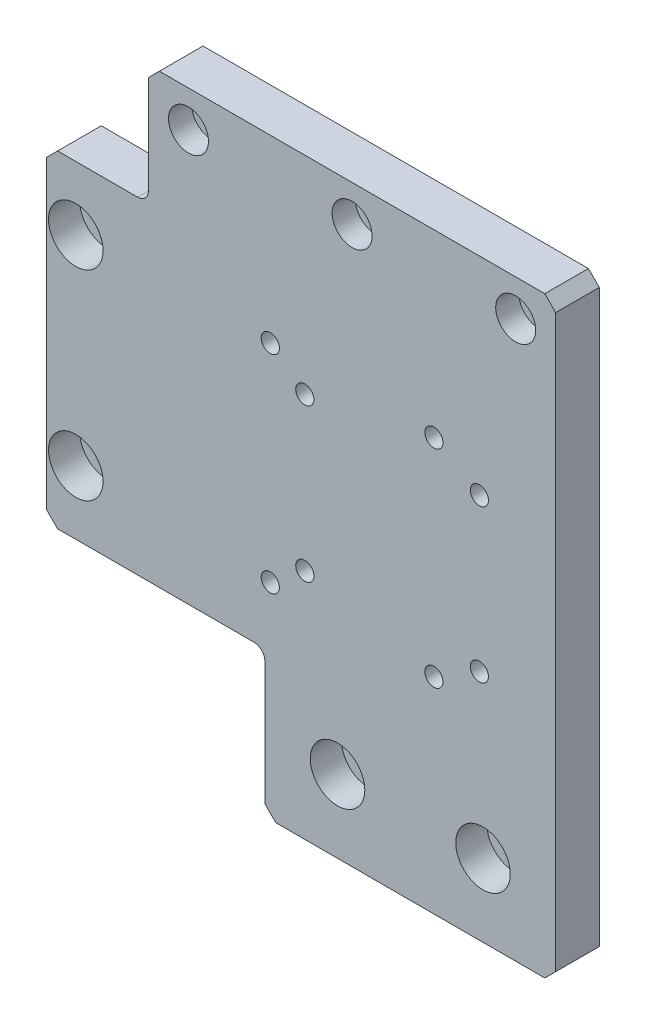
SolidWorks part; units mm, degrees
ref_plane "前视基准面" through (0, 0, 0) normal (0, 0, 1) x (1, 0, 0)
ref_plane "上视基准面" through (0, 0, 0) normal (0, 1, 0) x (1, 0, 0)
ref_plane "右视基准面" through (0, 0, 0) normal (1, 0, 0) x (0, 0, -1)
sketch "草图1" plane through (0, 0, 0) normal (0, 0, 1) x (1, 0, 0)
  line L1 (0, 0) -> (140, 0)
  line L2 (0, 0) -> (0, 112)
  line L3 (0, 112) -> (140, 112)
  line L4 (140, 0) -> (140, 112)
  dimension "D1" = 140
  dimension "D2" = 112
extrude "凸台-拉伸1" add sketch "草图1" along normal blind 12
hole_wizard "M6 螺纹孔1" positions "草图3" profile "草图2" tap size "M6" standard "ISO" end condition through all
sketch "草图3" plane through (0, 0, 0) normal (0, 0, -1) x (-1, 0, 0)
  point P0 (-106.5, 84.5)
  point P8 (-61.5, 84.5)
  point P11 (-61.5, 27.5)
  point P14 (-106.5, 27.5)
sketch "草图2" plane through (106.5, 84.5, 0) normal (1, 0, 0) x (0, 1, 0)
  line L0 (0, 0) -> (0, 12)
  line L1 (0, 12) -> (2.5, 12)
  line L2 (2.5, 12) -> (2.5, 0)
  line L5 (2.5, 0) -> (0, 0)
  line L11 (0, -6.35) -> (0, 107.95) construction
  dimension "通孔螺纹孔钻头直径" = 5
  dimension "通孔螺纹孔钻头深度" = 12
cosmetic thread "孔螺蚊线1" parameters "D2"=6
cosmetic thread "孔螺蚊线2" parameters "D2"=6
cosmetic thread "孔螺蚊线3" parameters "D2"=6
cosmetic thread "孔螺蚊线4" parameters "D2"=6
hole_wizard "M6 螺纹孔2" positions "草图5" profile "草图4" tap size "M6" standard "ISO" end condition through all
sketch "草图5" plane through (0, 0, 12) normal (0, 0, 1) x (1, 0, 0)
  circle A0 centre (119, 77) radius 3.3235 construction
  circle A1 centre (71, 77) radius 3.3235 construction
  circle A2 centre (119, 35) radius 3.3235 construction
  circle A3 centre (71, 35) radius 3.3235 construction
  point P0 (71, 77)
  point P3 (71, 35)
  point P6 (119, 35)
  point P9 (119, 77)
sketch "草图4" plane through (71, 77, 12) normal (1, 0, 0) x (0, -1, 0)
  line L0 (0, 0) -> (0, 12)
  line L1 (0, 12) -> (2.5, 12)
  line L2 (2.5, 12) -> (2.5, 0)
  line L5 (2.5, 0) -> (0, 0)
  line L11 (0, -6.35) -> (0, 107.95) construction
  dimension "通孔螺纹孔钻头直径" = 5
  dimension "通孔螺纹孔钻头深度" = 12
cosmetic thread "孔螺蚊线5"
cosmetic thread "孔螺蚊线6"
cosmetic thread "孔螺蚊线7"
cosmetic thread "孔螺蚊线8"
sketch "草图6" plane through (0, 112, 0) normal (0, 1, 0) x (1, 0, 0)
  line L0 (140, -12) -> (0, -12) construction
  line L1 (140, 0) -> (28, 0)
  line L2 (140, 0) -> (140, -12)
  line L3 (140, -12) -> (28, -12)
  line L4 (28, 0) -> (28, -12)
  dimension "D1" = 112
extrude "凸台-拉伸2" add sketch "草图6" along normal blind 22
sketch "草图7" plane through (0, 112, 0) normal (0, 1, 0) x (1, 0, 0)
  line L4 (28, -12) -> (28, 0)
  line L5 (28, 0) -> (0, 0)
  line L6 (0, 0) -> (0, -12)
  line L7 (0, -12) -> (28, -12)
  line L8 (28, -12) -> (28, 0)
  line L9 (28, 0) -> (0, 0)
  line L10 (0, 0) -> (0, -12)
  line L11 (0, -12) -> (28, -12)
  dimension "D1" = 0
extrude "切除-拉伸1" cut sketch "草图7" against normal blind 11
sketch "草图8" plane through (0, 0, 0) normal (0, -1, 0) x (1, 0, 0)
  line L0 (0, 12) -> (140, 12) construction
  line L1 (0, 0) -> (60, 0)
  line L2 (0, 0) -> (0, 12)
  line L3 (0, 12) -> (60, 12)
  line L4 (60, 0) -> (60, 12)
  dimension "D1" = 60
extrude "切除-拉伸2" cut sketch "草图8" against normal blind 11
hole_wizard "M6 六角凹头螺钉的柱形沉头孔1" positions "草图10" profile "草图9" counterbore size "M6" standard "ISO" end condition through all
sketch "草图10" plane through (0, 0, 12) normal (0, 0, 1) x (1, 0, 0)
  point P0 (129, 124)
  point P3 (84, 124)
  point P6 (39, 124)
sketch "草图9" plane through (129, 124, 12) normal (1, 0, 0) x (0, -1, 0)
  line L0 (0, 0) -> (0, 12)
  line L1 (0, 12) -> (3.3, 12)
  line L3 (3.3, 12) -> (3.3, 6.4)
  line L4 (3.3, 6.4) -> (5.5, 6.4)
  line L5 (5.5, 6.4) -> (5.5, 0)
  line L7 (5.5, 0) -> (0, 0)
  line L11 (0, -6.35) -> (0, 107.95) construction
  dimension "通孔孔直径" = 6.6
  dimension "通孔孔深度" = 12
  dimension "柱形沉头孔直径" = 11
  dimension "柱形沉头孔深度" = 6.4
sketch "草图11" plane through (0, 0, 0) normal (0, -1, 0) x (1, 0, 0)
  line L4 (140, 12) -> (60, 12)
  line L5 (60, 12) -> (60, 0)
  line L6 (60, 0) -> (140, 0)
  line L7 (140, 0) -> (140, 12)
  line L8 (140, 12) -> (60, 12)
  line L9 (60, 12) -> (60, 0)
  line L10 (60, 0) -> (140, 0)
  line L11 (140, 0) -> (140, 12)
  dimension "D1" = 0
extrude "凸台-拉伸3" add sketch "草图11" along normal blind 29
chamfer "倒角1" distance 3 angle 45 6 edges at (140, -29, 6) (60, -29, 6) (0, 11, 6) (140, 134, 6) (0, 101, 6) (28, 134, 6)
fillet "圆角1" radius 3 2 edges at (60, 11, 6) (28, 101, 6)
hole_wizard "M8 六角凹头螺钉的柱形沉头孔1" positions "草图14" profile "草图12" counterbore size "M8" standard "ISO" end condition through all
sketch "草图14" plane through (0, 0, 12) normal (0, 0, 1) x (1, 0, 0)
  point P0 (8, 83.5)
  point P3 (8, 28.5)
sketch "草图12" plane through (8, 83.5, 12) normal (1, 0, 0) x (0, -1, 0)
  line L0 (0, 0) -> (0, 12)
  line L1 (0, 12) -> (4.5, 12)
  line L3 (4.5, 12) -> (4.5, 8.6)
  line L4 (4.5, 8.6) -> (7.5, 8.6)
  line L5 (7.5, 8.6) -> (7.5, 0)
  line L7 (7.5, 0) -> (0, 0)
  line L11 (0, -6.35) -> (0, 107.95) construction
  dimension "通孔孔直径" = 9
  dimension "通孔孔深度" = 12
  dimension "柱形沉头孔直径" = 15
  dimension "柱形沉头孔深度" = 8.6
hole_wizard "M8 六角凹头螺钉的柱形沉头孔2" positions "草图16" profile "草图15" counterbore size "M8" standard "ISO" end condition through all
sketch "草图16" plane through (0, 0, 12) normal (0, 0, 1) x (1, 0, 0)
  line L0 (60, 8) -> (60, -26) construction
  line L1 (137, -29) -> (63, -29) construction
  point P0 (80, -9)
  point P2 (120, -9)
  dimension "D1" = 20
  dimension "D2" = 20
  dimension "D3" = 40
  dimension "D4" = 20
sketch "草图15" plane through (80, -9, 12) normal (1, 0, 0) x (0, -1, 0)
  line L0 (0, 0) -> (0, 12)
  line L1 (0, 12) -> (4.5, 12)
  line L3 (4.5, 12) -> (4.5, 8.6)
  line L4 (4.5, 8.6) -> (7.5, 8.6)
  line L5 (7.5, 8.6) -> (7.5, 0)
  line L7 (7.5, 0) -> (0, 0)
  line L11 (0, -6.35) -> (0, 107.95) construction
  dimension "通孔孔直径" = 9
  dimension "通孔孔深度" = 12
  dimension "柱形沉头孔直径" = 15
  dimension "柱形沉头孔深度" = 8.6
